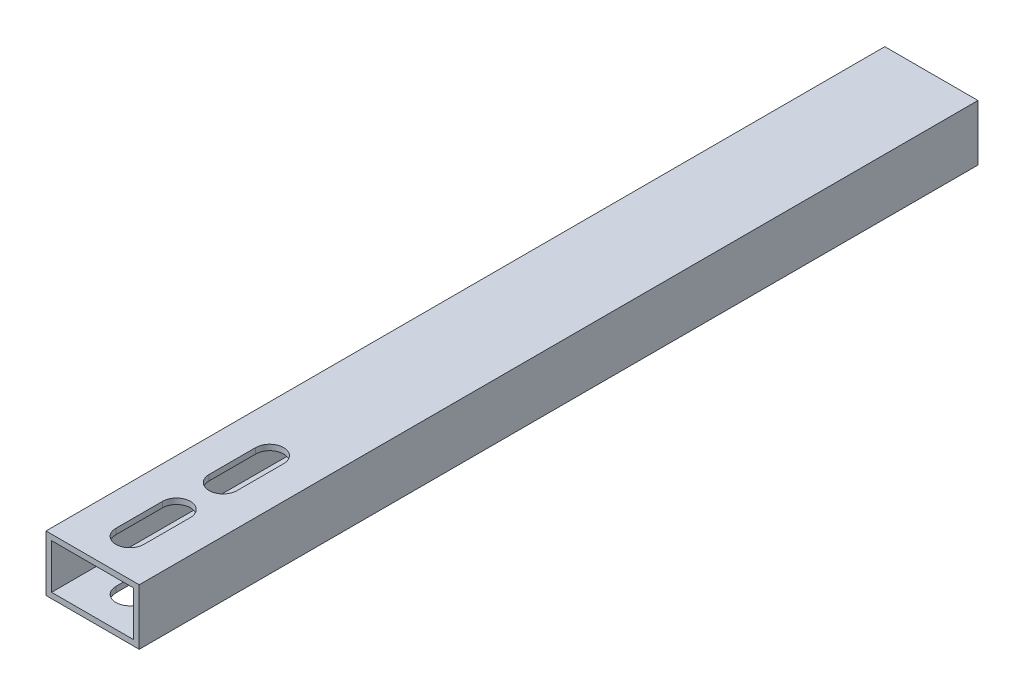
SolidWorks part; units mm, degrees
ref_plane "前视基准面" through (0, 0, 0) normal (0, 0, 1) x (1, 0, 0)
ref_plane "上视基准面" through (0, 0, 0) normal (0, 1, 0) x (1, 0, 0)
ref_plane "右视基准面" through (0, 0, 0) normal (1, 0, 0) x (0, 0, -1)
sketch "草图1" plane through (0, 0, 0) normal (0, 0, 1) x (1, 0, 0)
  line L0 (0, 0) -> (50, 0)
  line L1 (50, 0) -> (50, 30)
  line L2 (50, 30) -> (0, 30)
  line L3 (0, 30) -> (0, 0)
  line L4 (3, 3) -> (47, 3)
  line L5 (47, 3) -> (47, 27)
  line L6 (47, 27) -> (3, 27)
  line L7 (3, 27) -> (3, 3)
  dimension "D1" = 3
extrude "凸台-拉伸1" add sketch "草图1" along normal blind 450
sketch "草图2" plane through (0, 0, 0) normal (0, -1, 0) x (1, 0, 0)
  line L0 (17.5, 430) -> (17.5, 405)
  line L1 (32.5, 430) -> (32.5, 405)
  arc A0 (17.5, 405) -> (32.5, 405) centre (25, 405) ccw
  arc A3 (32.5, 430) -> (17.5, 430) centre (25, 430) ccw
extrude "切除-拉伸2" cut sketch "草图2" against normal blind 450
sketch "草图4" plane through (0, 0, 0) normal (0, -1, 0) x (1, 0, 0)
  line L0 (17.5, 380) -> (17.5, 355)
  line L3 (32.5, 380) -> (32.5, 355)
  arc A2 (32.5, 380) -> (17.5, 380) centre (25, 380) ccw
  arc A3 (17.5, 355) -> (32.5, 355) centre (25, 355) ccw
extrude "切除-拉伸3" cut sketch "草图4" against normal blind 450
